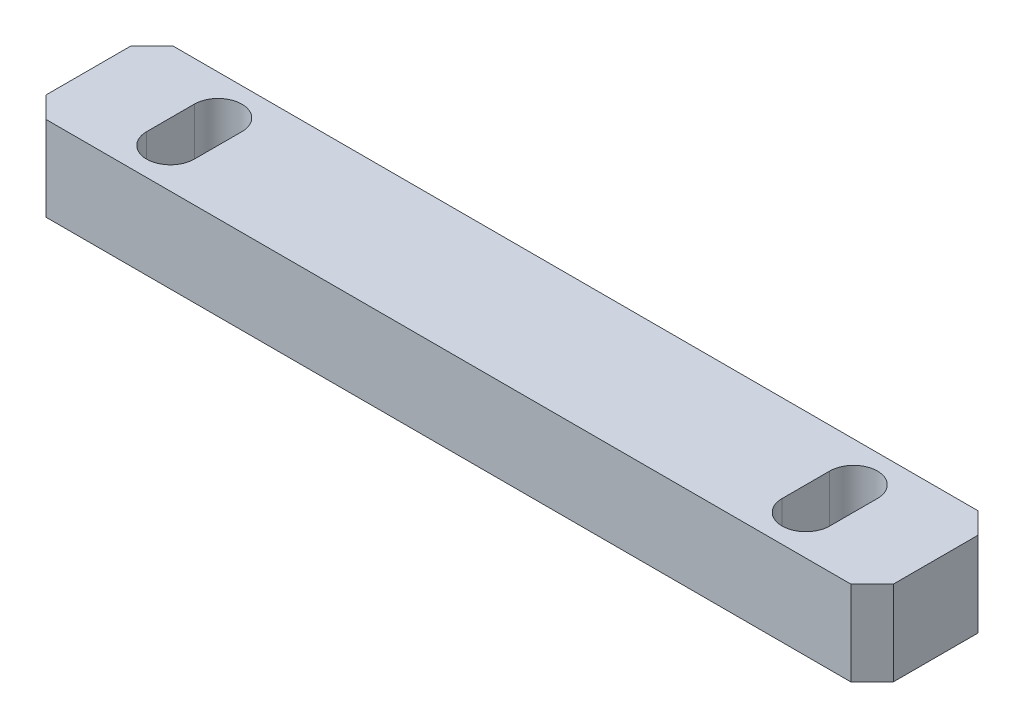
SolidWorks part; units mm, degrees
ref_plane "Front Plane" through (0, 0, 0) normal (0, 0, 1) x (1, 0, 0)
ref_plane "Top Plane" through (0, 0, 0) normal (0, 1, 0) x (1, 0, 0)
ref_plane "Right Plane" through (0, 0, 0) normal (1, 0, 0) x (0, 0, -1)
sketch "Sketch1" plane through (0, 0, 0) normal (0, 1, 0) x (1, 0, 0)
  line L1 (0, 0) -> (80, 0)
  line L2 (0, 0) -> (0, 12)
  line L3 (0, 12) -> (80, 12)
  line L4 (80, 0) -> (80, 12)
  dimension "D1" = 12
  dimension "D2" = 80
extrude "Boss-Extrude1" add sketch "Sketch1" along normal blind 8
chamfer "Chamfer1" distance 2 angle 45 4 edges at (0, 4, 0) (0, 4, -12) (80, 4, 0) (80, 4, -12)
sketch "Sketch2" plane through (0, 0, 0) normal (0, -1, 0) x (1, 0, 0)
  line L0 (40, -12) -> (40, 49988) construction
  line L1 (78, -12) -> (2, -12) construction
  line L2 (0, -6) -> (50000, -6) construction
  line L3 (0, -10) -> (0, -2) construction
  circle A0 centre (10, -6) radius 2.25
  circle A1 centre (70, -6) radius 2.25
  point P4 (40, -12)
  point P9 (0, -6)
  dimension "D1" = 60
  dimension "D2" = 4.5
extrude "Cut-Extrude1" cut sketch "Sketch2" against normal blind 10
sketch "Sketch4" plane through (0, 0, 0) normal (0, -1, 0) x (1, 0, 0)
  line L0 (10, -8.25) -> (10, -3.75) construction
  line L1 (7.75, -8.25) -> (7.75, -3.75)
  line L2 (12.25, -8.25) -> (12.25, -3.75)
  line L3 (40, 0) -> (40, -50000) construction
  line L4 (2, 0) -> (78, 0) construction
  line L5 (70, -8.25) -> (70, -3.75) construction
  line L6 (72.25, -8.25) -> (72.25, -3.75)
  line L7 (67.75, -8.25) -> (67.75, -3.75)
  circle A0 centre (10, -6) radius 2.25 construction
  arc A1 (7.75, -8.25) -> (12.25, -8.25) centre (10, -8.25) ccw
  arc A2 (12.25, -3.75) -> (7.75, -3.75) centre (10, -3.75) ccw
  arc A3 (72.25, -8.25) -> (67.75, -8.25) centre (70, -8.25) cw
  arc A4 (67.75, -3.75) -> (72.25, -3.75) centre (70, -3.75) cw
  point P5 (10, -6)
  point P14 (40, 0)
  point P17 (70, -6)
  dimension "D1" = 4.5
extrude "Cut-Extrude2" cut sketch "Sketch4" against normal blind 10
